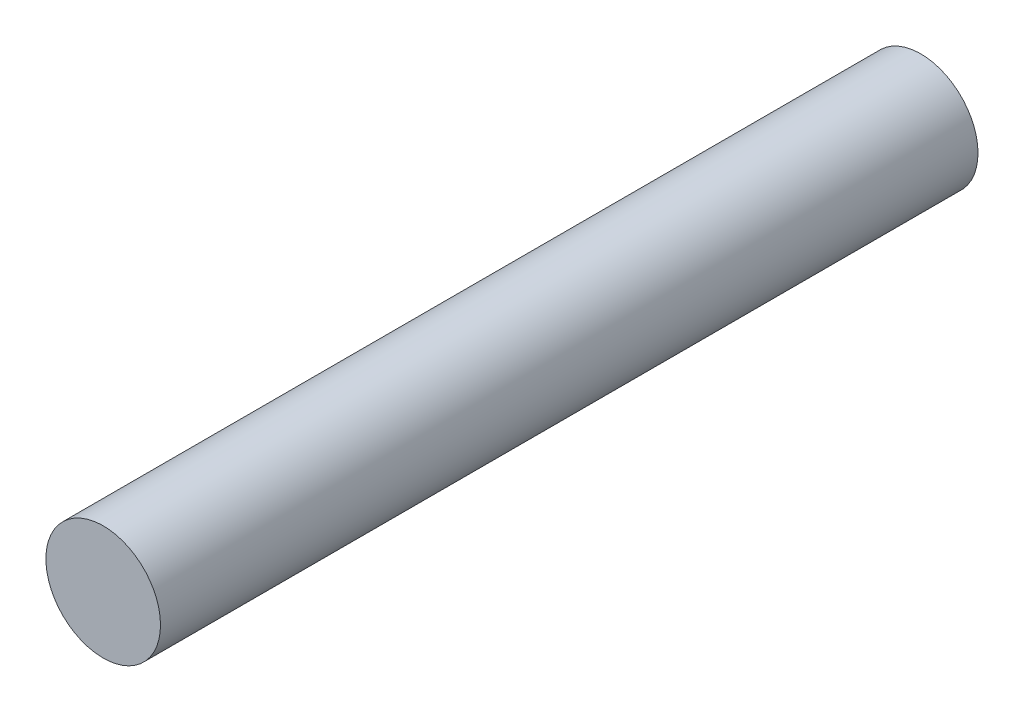
from build123d import *

# Parameters (mm, degrees)
BOSS_EXTRUDE1_DEPTH      = 94
BOSS_EXTRUDE1_DEPTH_BACK = 13
SKETCH1_R                = 7.5


with BuildPart() as part:
    # Sketch1 → Boss-Extrude1 (new, two sides: drawn at the far end of the back side and taken through both)
    with BuildSketch(Plane.XY.offset(-BOSS_EXTRUDE1_DEPTH_BACK)):
        Circle(SKETCH1_R)
    extrude(amount=BOSS_EXTRUDE1_DEPTH + BOSS_EXTRUDE1_DEPTH_BACK)


solid = part.part
